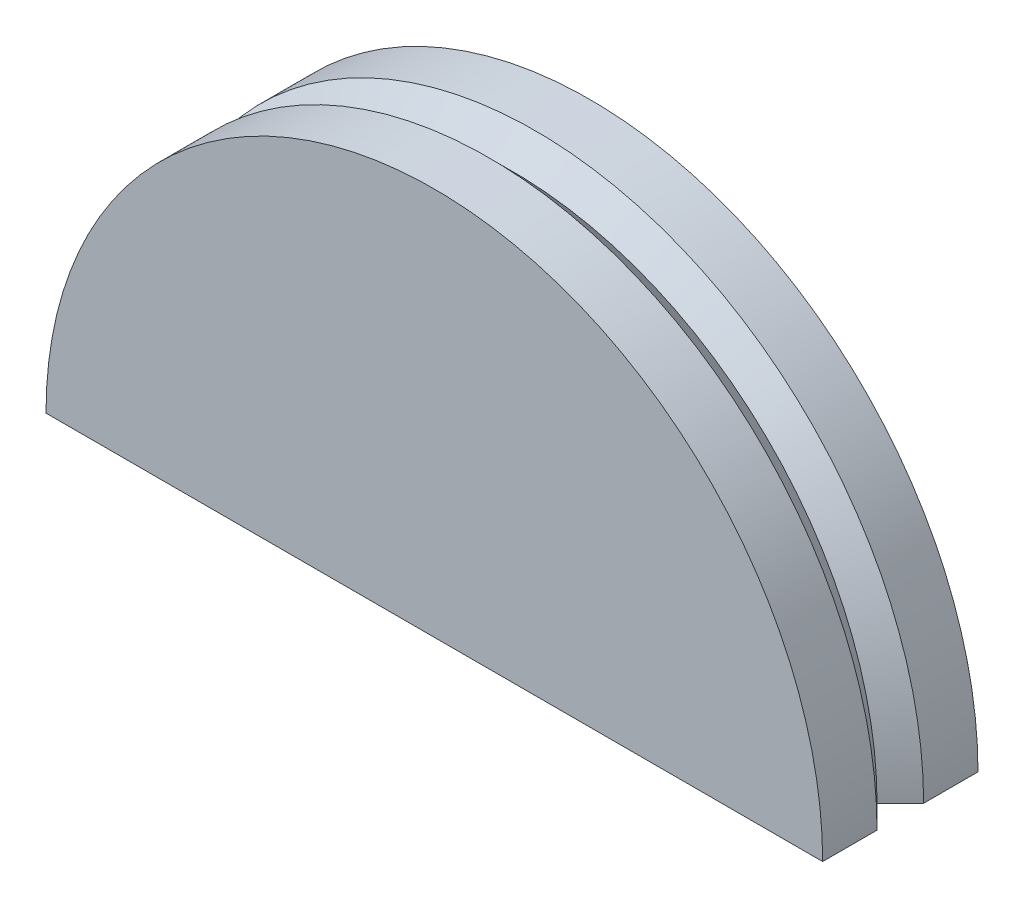
from build123d import *

# Parameters (mm, degrees)
BOSS_EXTRUDE1_DEPTH = 10


with BuildPart() as part:
    # Sketch1 → Boss-Extrude1 (new body)
    with BuildSketch(Plane.XY):
        with BuildLine():
            Line((-23.745241043, -21.468300121), (26.254758957, -21.468300121))
            ThreePointArc((26.254758957, -21.468300121), (1.254758957, 3.531699879), (-23.745241043, -21.468300121))
        make_face()
    extrude(amount=BOSS_EXTRUDE1_DEPTH)

    # Cut-Sweep1: sweep along a path in Sketch4
    with BuildLine(Plane.XY.offset(5)) as cut_sweep1_path:
        ThreePointArc((26.254758957, -21.468300121), (1.254758957, 3.531699879), (-23.745241043, -21.468300121))
    # Sketch2 → Cut-Sweep1 (sweep, cut)
    with BuildSketch(Plane.XZ.offset(21.468300121)):
        Polygon((26.254758957, 5), (26.254758957, 6.5), (24.754758957, 5), (26.254758957, 3.5), align=None)
    sweep(path=cut_sweep1_path.line, mode=Mode.SUBTRACT)


solid = part.part
